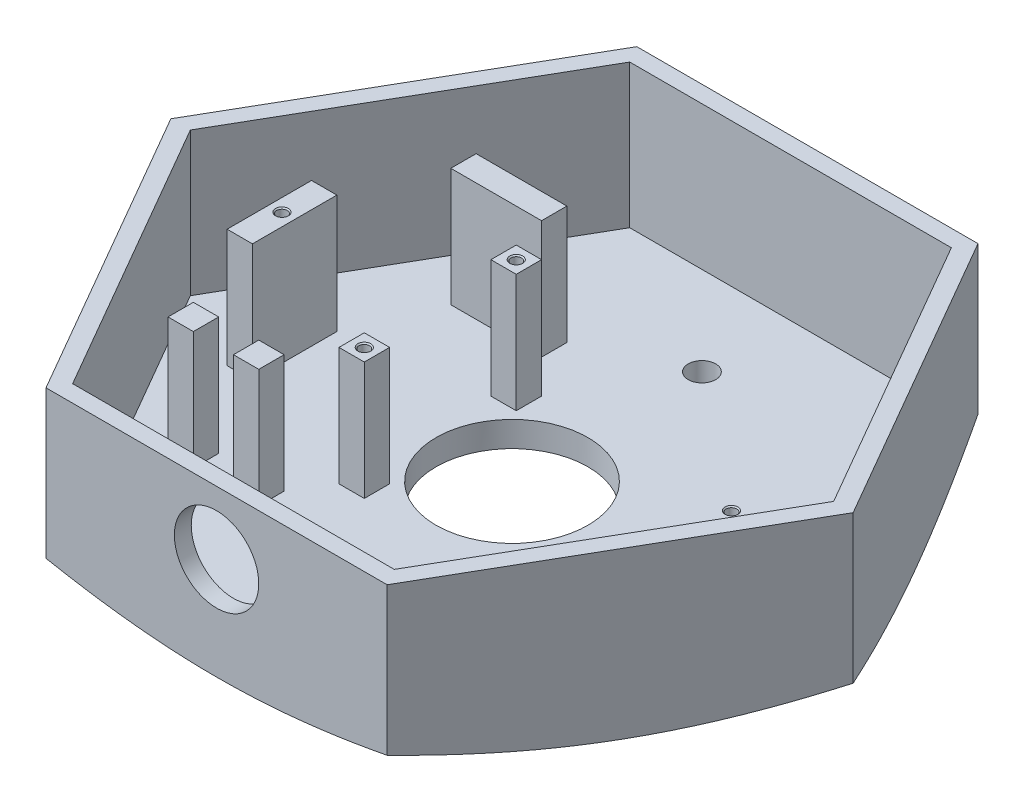
SolidWorks part; units mm, degrees
ref_plane "Front Plane" through (0, 0, 0) normal (0, 0, 1) x (1, 0, 0)
ref_plane "Top Plane" through (0, 0, 0) normal (0, 1, 0) x (1, 0, 0)
ref_plane "Right Plane" through (0, 0, 0) normal (1, 0, 0) x (0, 0, -1)
other "Configuration Table"
sketch "Sketch1" plane through (0, 0, 0) normal (0, 1, 0) x (1, 0, 0)
  line L1 (-40.4145, 70) -> (-80.829, 0)
  line L2 (-80.829, 0) -> (-40.4145, -70)
  line L3 (-40.4145, -70) -> (40.4145, -70)
  line L4 (40.4145, -70) -> (80.829, 0)
  line L5 (80.829, 0) -> (40.4145, 70)
  line L6 (40.4145, 70) -> (-40.4145, 70)
  circle A0 centre (0, 0) radius 70 construction
  dimension "D1" = 140
extrude "Boss-Extrude1" add sketch "Sketch1" along normal blind 41
sketch "Sketch2" plane through (0, 41, 0) normal (0, 1, 0) x (1, 0, 0)
  line L0 (38.1051, 66) -> (-38.1051, 66)
  line L1 (-38.1051, 66) -> (-76.2102, 0)
  line L2 (-76.2102, 0) -> (-38.1051, -66)
  line L3 (-38.1051, -66) -> (38.1051, -66)
  line L4 (38.1051, -66) -> (76.2102, 0)
  line L5 (76.2102, 0) -> (38.1051, 66)
  line L6 (40.4145, 70) -> (-40.4145, 70)
  line L7 (-40.4145, 70) -> (-80.829, 0)
  line L8 (-80.829, 0) -> (-40.4145, -70)
  line L9 (-40.4145, -70) -> (40.4145, -70)
  line L10 (40.4145, -70) -> (80.829, 0)
  line L11 (80.829, 0) -> (40.4145, 70)
  line L12 (40.4145, 70) -> (-40.4145, 70)
  line L14 (-80.829, 0) -> (-40.4145, -70)
  line L15 (-40.4145, -70) -> (40.4145, -70)
  line L16 (40.4145, -70) -> (80.829, 0)
  line L17 (80.829, 0) -> (40.4145, 70)
  line L18 (-40.4145, 70) -> (-80.829, 0) construction
  dimension "D1" = 0
  dimension "D2" = 4
extrude "Cut-Extrude1" cut sketch "Sketch2" against normal blind 34 contours L4 L5 L0 L1 L2 L3
sketch "Sketch3" plane through (0, 0, 0) normal (0, 0, 1) x (1, 0, 0)
  line L0 (0, 62.9006) -> (0, 0) construction
  line L1 (-80.829, 6) -> (-65.1985, 0)
  line L2 (-80.829, 41) -> (-80.829, 0) construction
  line L3 (-80.829, 0) -> (-40.4145, 0) construction
  line L4 (-65.1985, 0) -> (-80.829, 0)
  line L5 (-80.829, 0) -> (-80.829, 6)
  line L6 (-80.829, 41) -> (-40.4145, 41) construction
  dimension "D1" = 35
  dimension "D2" = 21
revolve "Cut-Revolve1" cut sketch "Sketch3" angle 360 about L0
sketch "Sketch4" plane through (0, 0, 0) normal (0, -1, 0) x (1, 0, 0)
  circle A0 centre (0, 0) radius 52.5
  dimension "D1" = 105
extrude "Cut-Extrude2" cut sketch "Sketch4" against normal blind 1
sketch "Sketch5" plane through (0, 7, 0) normal (0, 1, 0) x (1, 0, 0)
  line L0 (0, 103.6937) -> (0, 0) construction
  line L1 (-43.5, 35) -> (-22, 35)
  line L2 (-43.5, 35) -> (-43.5, 29)
  line L3 (-43.5, 29) -> (-22, 29)
  line L4 (-22, 35) -> (-22, 29)
  line L5 (-43.5, 35) -> (-22, 29) construction
  line L6 (-43.5, 29) -> (-22, 35) construction
  line L7 (-57.5, 10) -> (-51.5, 10)
  line L8 (-57.5, 10) -> (-57.5, -10)
  line L9 (-57.5, -10) -> (-51.5, -10)
  line L10 (-51.5, 10) -> (-51.5, -10)
  line L11 (-57.5, 10) -> (-51.5, -10) construction
  line L12 (-57.5, -10) -> (-51.5, 10) construction
  line L13 (-46.5, -29) -> (-40.5, -29)
  line L14 (-46.5, -29) -> (-46.5, -35)
  line L15 (-46.5, -35) -> (-40.5, -35)
  line L16 (-40.5, -29) -> (-40.5, -35)
  line L17 (-46.5, -29) -> (-40.5, -35) construction
  line L18 (-46.5, -35) -> (-40.5, -29) construction
  line L19 (-31, -29) -> (-25, -29)
  line L20 (-31, -29) -> (-31, -35)
  line L21 (-31, -35) -> (-25, -35)
  line L22 (-25, -29) -> (-25, -35)
  line L23 (-31, -29) -> (-25, -35) construction
  line L24 (-31, -35) -> (-25, -29) construction
  line L25 (-20, 21) -> (-14, 21)
  line L26 (-20, 21) -> (-20, 15)
  line L27 (-20, 15) -> (-14, 15)
  line L28 (-14, 21) -> (-14, 15)
  line L29 (-20, 21) -> (-14, 15) construction
  line L30 (-20, 15) -> (-14, 21) construction
  line L31 (0, 0) -> (-91.501, 0) construction
  line L32 (-43.5, -32) -> (-28, -32) construction
  line L33 (-28, -32) -> (0, -32) construction
  line L34 (0, -32) -> (0, 0) construction
  line L35 (-20, -15) -> (-14, -21) construction
  line L36 (-20, -21) -> (-14, -15) construction
  line L37 (-14, -21) -> (-14, -15)
  line L38 (-20, -15) -> (-14, -15)
  line L39 (-20, -21) -> (-20, -15)
  line L40 (-20, -21) -> (-14, -21)
  point P0 (-32.75, 32)
  point P5 (-54.5, 0)
  point P10 (-43.5, -32)
  point P15 (-28, -32)
  point P20 (-17, 18)
  point P36 (-17, -18)
  dimension "D1" = 21.5
  dimension "D2" = 5
  dimension "D3" = 17
  dimension "D4" = 32
  dimension "D5" = 36
  dimension "D6" = 6
  dimension "D7" = 6
  dimension "D8" = 6
  dimension "D9" = 6
  dimension "D10" = 20
  dimension "D11" = 54.5
  dimension "D12" = 6
  dimension "D13" = 6
  dimension "D14" = 6
  dimension "D15" = 6
  dimension "D16" = 28
  dimension "D17" = 15.5
  dimension "D18" = 32
extrude "Boss-Extrude2" add sketch "Sketch5" along normal blind 28
sketch "Sketch6" plane through (0, 7, 0) normal (0, 1, 0) x (1, 0, 0)
  circle A0 centre (0, 0) radius 18
  dimension "D1" = 36
extrude "Cut-Extrude3" cut sketch "Sketch6" against normal blind 28
sketch "Sketch7" plane through (0, 7, 0) normal (0, 1, 0) x (1, 0, 0)
  line L0 (0, 45) -> (0, 0) construction
  line L1 (0, 0) -> (-24.165, 0) construction
  circle A0 centre (0, 45) radius 3.25
  circle A1 centre (0, -45) radius 3.25
  dimension "D2" = 6.5
  dimension "D1" = 45
extrude "Cut-Extrude4" cut sketch "Sketch7" against normal blind 28
sketch "Sketch8" plane through (0, 0, 66) normal (0, 0, -1) x (-1, 0, 0)
  line L0 (0, 26) -> (0, 0) construction
  line L1 (-40.4145, 41) -> (40.4145, 41) construction
  circle A0 centre (0, 26) radius 10
  dimension "D2" = 20
  dimension "D1" = 15
sketch "Sketch9" plane through (0, 7, 0) normal (0, 1, 0) x (1, 0, 0)
  line L0 (0, 0) -> (32, 0) construction
  line L1 (32, 0) -> (32, 20) construction
  point P4 (32, -20)
  point P5 (32, 20)
  dimension "D1" = 32
  dimension "D2" = 40
hole_wizard "M3 Tapped Hole1" positions "Sketch9" profile "Sketch10" tap size "M3" standard "GB" end condition through all
sketch "Sketch10" plane through (32, 7, -20) normal (1, 0, 0) x (0, 0, 1)
  line L0 (0, 0) -> (0, 7)
  line L1 (0, 7) -> (1.25, 7)
  line L2 (1.25, 7) -> (1.25, 0.275)
  line L3 (1.25, 0.275) -> (1.525, 0)
  line L5 (1.525, 0) -> (0, 0)
  line L6 (-1.25, 0.275) -> (-1.525, 0) construction
  line L11 (0, -6.35) -> (0, 107.95) construction
  dimension "通孔螺纹孔钻头直径" = 2.5
  dimension "通孔螺纹孔钻头深度" = 7
  dimension "近端锥形沉头孔直径" = 3.05
  dimension "近端锥形沉头孔角度" = 90
cosmetic thread "Hole cosmetic thread1" parameters "D2"=3
cosmetic thread "Hole cosmetic thread2" parameters "D2"=3
sketch "Sketch11" plane through (0, 35, 0) normal (0, 1, 0) x (1, 0, 0)
  line L0 (-17, 21) -> (-17, -21) construction
  line L1 (-14, 21) -> (-20, 21) construction
  line L2 (-20, -21) -> (-14, -21) construction
  line L3 (-14, 18) -> (-20, 18) construction
  line L4 (-14, 15) -> (-14, 21) construction
  line L5 (-20, 21) -> (-20, 15) construction
  line L6 (-14, -18) -> (-20, -18) construction
  line L7 (-14, -21) -> (-14, -15) construction
  line L8 (-20, -15) -> (-20, -21) construction
  line L9 (0, 0) -> (-54.5, 0) construction
  line L10 (-54.5, 0) -> (-54.5, 10) construction
  line L11 (-51.5, 10) -> (-57.5, 10) construction
  point P18 (-17, 18)
  point P19 (-17, -18)
  point P27 (-54.5, 0)
hole_wizard "M3 Tapped Hole2" positions "Sketch11" profile "Sketch12" tap size "M3" standard "GB"
cosmetic thread "Hole cosmetic thread3" parameters "D1"=4, "D2"=3
cosmetic thread "Hole cosmetic thread4" parameters "D1"=4, "D2"=3
cosmetic thread "Hole cosmetic thread5" parameters "D1"=4, "D2"=3
sketch "Sketch12" plane through (-54.5, 35, 0) normal (1, 0, 0) x (0, 0, 1)
  line L0 (0, 0) -> (0, 8.7511)
  line L1 (0, 8.7511) -> (1.25, 8)
  line L2 (1.25, 8) -> (1.25, 0.275)
  line L3 (1.25, 0.275) -> (1.525, 0)
  line L5 (1.525, 0) -> (0, 0)
  line L6 (-1.25, 0.275) -> (-1.525, 0) construction
  line L10 (0, 8.7511) -> (-1.25, 8) construction
  line L11 (0, -6.35) -> (0, 107.95) construction
  dimension "螺纹孔钻头直径" = 2.5
  dimension "螺纹孔钻头深度" = 8
  dimension "近端锥形沉头孔直径" = 3.05
  dimension "近端锥形沉头孔角度" = 90
  dimension "导头角度" = 118
extrude "Cut-Extrude5" cut sketch "Sketch8" against normal blind 28
